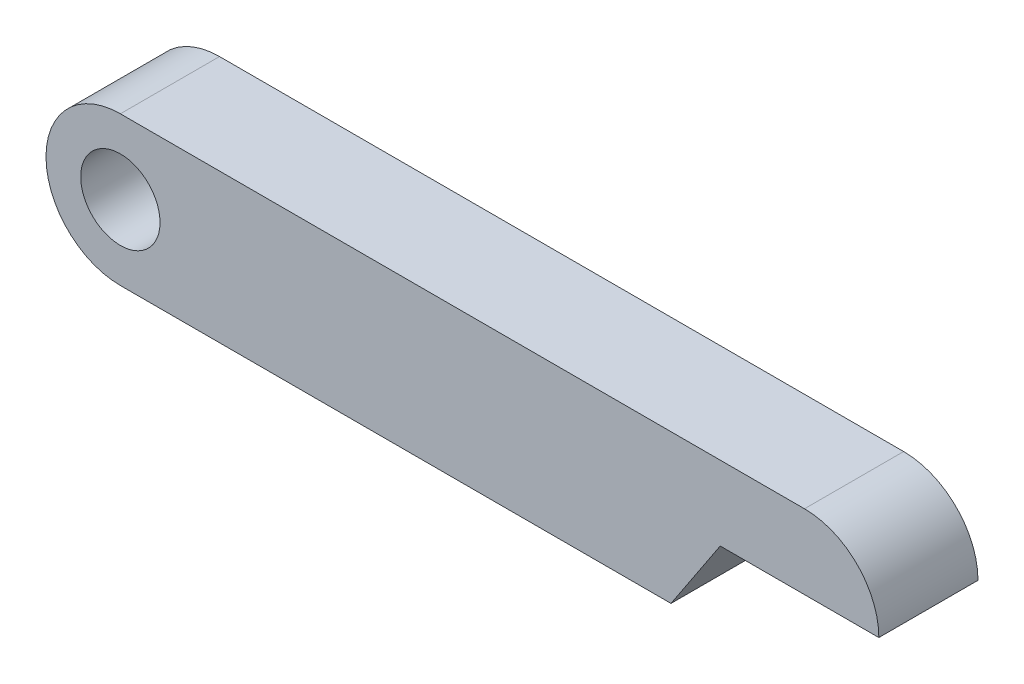
from build123d import *

# Parameters (mm, degrees)
SKETCH1_R           = 4
BOSS_EXTRUDE1_DEPTH = 10


with BuildPart() as part:
    # Sketch1 → Boss-Extrude1 (new body)
    with BuildSketch(Plane.XY):
        with BuildLine():
            Line((0, 7.5), (69, 7.5))
            ThreePointArc((69, 7.5), (74.303300859, 5.303300859), (76.5, 0))
            Line((76.5, 0), (60.5, 0))
            Line((60.5, 0), (55.535633926, -7.5))
            Line((55.535633926, -7.5), (0, -7.5))
            ThreePointArc((0, -7.5), (-7.5, 0), (0, 7.5))
        make_face()
        Circle(SKETCH1_R, mode=Mode.SUBTRACT)
    extrude(amount=BOSS_EXTRUDE1_DEPTH)


solid = part.part
